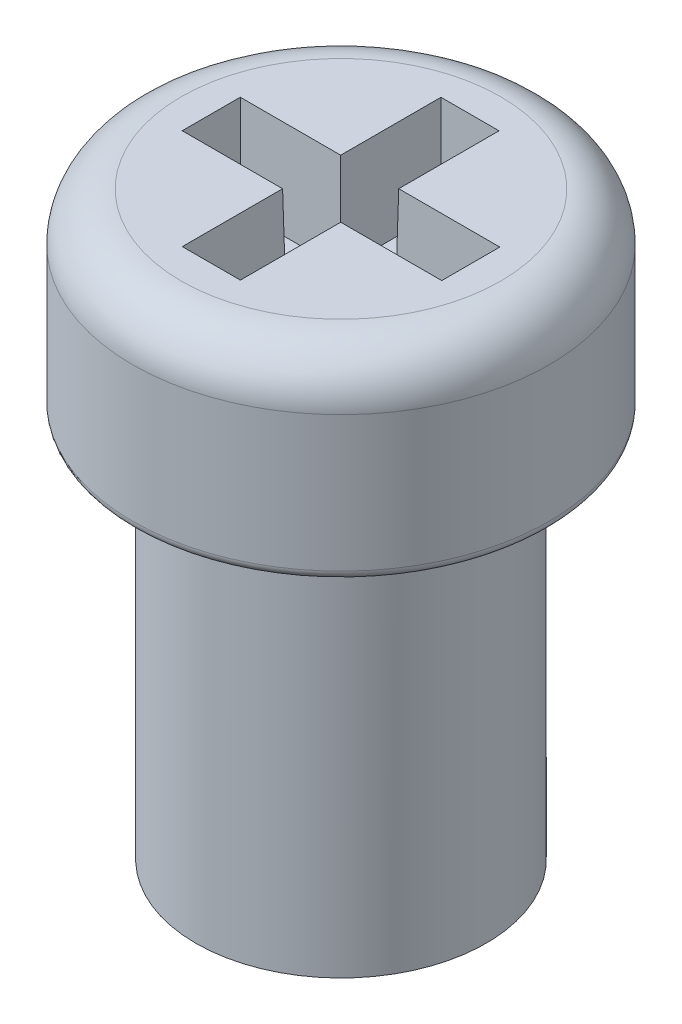
from build123d import *

# Parameters (mm, degrees)
SKETCH1_R           = 2.15
BOSS_EXTRUDE1_DEPTH = 2
SKETCH2_R           = 1.5
BOSS_EXTRUDE2_DEPTH = 4
FILLET1_R           = 0.5
FILLET2_R           = 0.1
CUT_EXTRUDE1_DEPTH  = 1
CUT_EXTRUDE1_DRAFT  = -1


with BuildPart() as part:
    # Sketch1 → Boss-Extrude1 (new body)
    with BuildSketch(Plane(origin=(0, 0, 0), x_dir=(1, 0, 0), z_dir=(0, 1, 0))):
        with Locations(Location((0, 0, 0), (0, 0, 270))):
            Circle(SKETCH1_R)
    extrude(amount=BOSS_EXTRUDE1_DEPTH)

    # Sketch2 → Boss-Extrude2 (add)
    with BuildSketch(Plane.XZ):
        with Locations(Location((0, 0, 0), (0, 0, 90))):
            Circle(SKETCH2_R)
    extrude(amount=BOSS_EXTRUDE2_DEPTH)

    # Fillet1
    fillet1_edges = [part.edges().sort_by_distance(p)[0] for p in [
        (0, 2, -2.15),
    ]]
    fillet(fillet1_edges, radius=FILLET1_R)

    # Fillet2
    fillet2_edges = [part.edges().sort_by_distance(p)[0] for p in [
        (0, 0, -2.15),
    ]]
    fillet(fillet2_edges, radius=FILLET2_R)


with BuildPart() as cut_extrude1_tool:
    # Sketch3 → Cut-Extrude1 (with draft: the straight prism first)
    with BuildSketch(Plane(origin=(0, 2, 0), x_dir=(1, 0, 0), z_dir=(0, 1, 0))):
        Polygon((0.296573117, 0.3), (0.296573117, 1.336133674), (-0.303426883, 1.336133674), (-0.303426883, 0.3), (-1.340662941, 0.3), (-1.340662941, -0.3), (-0.303426883, -0.3), (-0.303426883, -1.336133674), (0.296573117, -1.336133674), (0.296573117, -0.3), (1.340662941, -0.3), (1.340662941, 0.3), align=None)
    extrude(amount=-CUT_EXTRUDE1_DEPTH)
    # Cut-Extrude1: the draft: its side faces are tilted about the plane it starts from
    cut_extrude1_sides = [cut_extrude1_tool.faces().sort_by_distance(p)[0] for p in [
        (0.296573117, 1.5, -0.818066837),
        (-0.003426883, 1.5, -1.336133674),
        (-0.303426883, 1.5, -0.818066837),
        (-0.822044912, 1.5, -0.3),
        (-1.340662941, 1.5, 0),
        (-0.822044912, 1.5, 0.3),
        (-0.303426883, 1.5, 0.818066837),
        (-0.003426883, 1.5, 1.336133674),
        (0.296573117, 1.5, 0.818066837),
        (0.818618029, 1.5, 0.3),
        (1.340662941, 1.5, 0),
        (0.818618029, 1.5, -0.3),
    ]]
    draft(cut_extrude1_sides, Plane(origin=(0, 2, 0), x_dir=(1, 0, 0), z_dir=(0, 1, 0)), CUT_EXTRUDE1_DRAFT)


with BuildPart() as part_1:
    add(part.part)

    # Cut-Extrude1: cut by cut_extrude1_tool
    add(cut_extrude1_tool.part, mode=Mode.SUBTRACT)


solid = part_1.part
